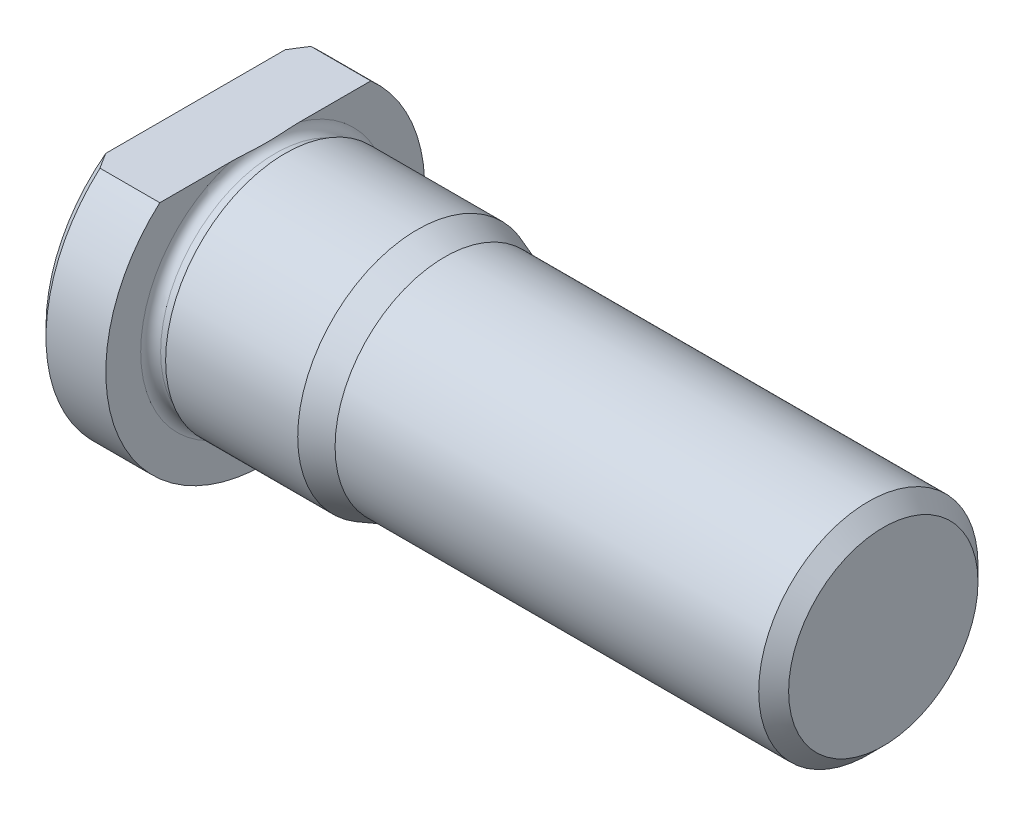
SolidWorks part; units mm, degrees
material "普通碳钢"
ref_plane "前视" through (0, 0, 0) normal (0, 0, 1) x (1, 0, 0)
ref_plane "上视" through (0, 0, 0) normal (0, 1, 0) x (1, 0, 0)
ref_plane "右视" through (0, 0, 0) normal (1, 0, 0) x (0, 0, -1)
sketch "草图1" plane through (0, 0, 0) normal (0, 0, 1) x (1, 0, 0)
  line L0 (-47.6935, 0) -> (46.0996, 0) construction
  line L1 (0, 30.9579) -> (0, -29.1188) construction
  line L2 (0, 0) -> (0, 16)
  line L3 (0, 16) -> (7, 16)
  line L4 (7, 16) -> (7, 11.5)
  line L5 (7, 11.5) -> (9, 11.5)
  line L6 (9, 11.5) -> (9, 12)
  line L7 (9, 12) -> (22.2525, 12)
  line L9 (25, 11) -> (69, 11)
  line L10 (69, 11) -> (69, 0)
  line L11 (69, 0) -> (0, 0)
  line L12 (25, 11) -> (22.2525, 12)
  dimension "D1" = 32
  dimension "D2" = 24
  dimension "D3" = 7
  dimension "22" = 22
  dimension "D4" = 18
  dimension "D5" = 69
  dimension "D6" = 23
  dimension "D7" = 2
  dimension "D8" = 20
revolve "旋转1" add sketch "草图1" angle 360 about L0
chamfer "倒角1" distance 1 angle 45 1 edges at (0, 0, 16)
fillet "圆角1" radius 1 1 edges at (7, 0, 11.5)
chamfer "倒角3" distance 1.5 angle 45 1 edges at (69, 0, 11)
sketch "草图2" plane through (0, 0, 0) normal (1, 0, 0) x (0, 0, -1)
  line L0 (-10.583, 12) -> (10.583, 12)
  line L1 (50, 0) -> (-50, 0) construction
  arc A0 (10.583, 12) -> (-10.583, 12) centre (0, 0) ccw
  dimension "D1" = 12
  dimension "D2" = 32
extrude "切除-拉伸5" cut sketch "草图2" along normal blind 8
